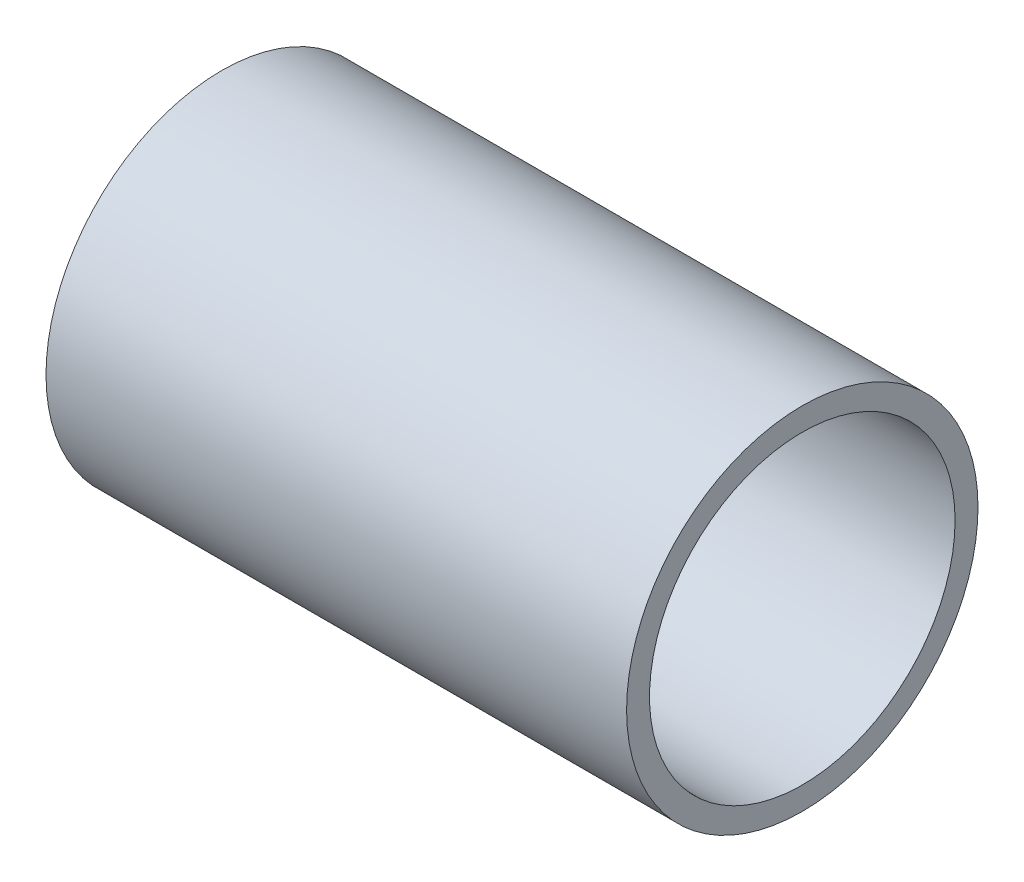
from build123d import *

# Parameters (mm, degrees)
SKETCH_1_R      = 23
SKETCH_1_R_2    = 20
EXTRUDE_1_DEPTH = 76


with BuildPart() as part:
    # 草图1 → 凸台-拉伸1 (new body)
    with BuildSketch(Plane(origin=(0, 0, 0), x_dir=(0, 0, -1), z_dir=(1, 0, 0))):
        Circle(SKETCH_1_R)
        Circle(SKETCH_1_R_2, mode=Mode.SUBTRACT)
    extrude(amount=EXTRUDE_1_DEPTH)


solid = part.part
